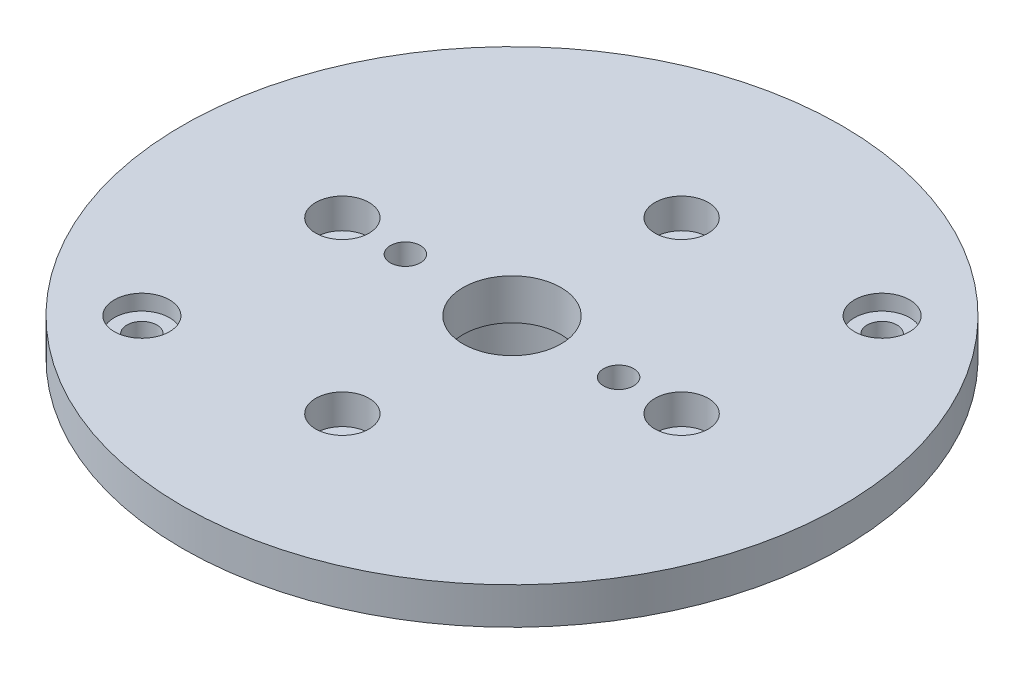
from build123d import *

# Parameters (mm, degrees)
SKETCH1_R               = 20
SKETCH1_R_2             = 7.5
BOSS_EXTRUDE1_DEPTH     = 12
SKETCH9_W               = 1.3
SKETCH9_H               = 0.7
SKETCH12_W              = 14
SKETCH12_H              = 3.8
SKETCH5_R               = 0.8
CUT_EXTRUDE2_DEPTH      = 50.558046773
SKETCH11_R              = 2.75
SKETCH11_R_2            = 1.5
CUT_EXTRUDE4_DEPTH      = 3.1
SKETCH14_W              = 4.95
SKETCH14_H              = 4.2
CUT_EXTRUDE5_DEPTH      = 50.558046773
CUT_EXTRUDE5_DEPTH_BACK = 1.6
SKETCH15_R              = 2.85
SKETCH7_R               = 1.55
CUT_EXTRUDE3_DEPTH      = 3
SKETCH16_R              = 1.55
CUT_EXTRUDE6_DEPTH      = 50.195121709
SKETCH17_R              = 1.55
CUT_EXTRUDE7_DEPTH      = 50.195121709
SKETCH18_R              = 1.5
CUT_EXTRUDE8_DEPTH      = 50.558046773


with BuildPart() as part:
    # Sketch1 → Boss-Extrude1 (new body)
    with BuildSketch(Plane(origin=(0, 0, 0), x_dir=(1, 0, 0), z_dir=(0, 1, 0))):
        with Locations(Location((0, 0, 0), (0, 0, 270))):
            Circle(SKETCH1_R)
        with Locations(Location((0, 0, 0), (0, 0, 270))):
            Circle(SKETCH1_R_2, mode=Mode.SUBTRACT)
    extrude(amount=BOSS_EXTRUDE1_DEPTH)

    # Sketch9 → Cut-Revolve3 (revolve, cut)
    with BuildSketch(Plane.XY, mode=Mode.PRIVATE) as cut_revolve3_sk:
        with Locations((14.4, 0.35)):
            Rectangle(SKETCH9_W, SKETCH9_H)
    revolve(cut_revolve3_sk.sketch.rotate(Axis((0, -3.122441051, 0), (0, 1, 0)), 90), axis=Axis((0, -3.122441051, 0), (0, 1, 0)), mode=Mode.SUBTRACT)

    # Sketch12 → Revolve1 (revolve)
    with BuildSketch(Plane.XY, mode=Mode.PRIVATE) as revolve1_sk:
        with Locations((27, 10.1)):
            Rectangle(SKETCH12_W, SKETCH12_H)
    revolve(revolve1_sk.sketch.rotate(Axis((0, 0, 0), (0, 1, 0)), 90), axis=Axis((0, 0, 0), (0, 1, 0)))

    # Sketch5 → Cut-Extrude2 (cut, through all)
    with BuildSketch(Plane(origin=(0, 12, 0), x_dir=(1, 0, 0), z_dir=(0, 1, 0))):
        with Locations(Location((11, 0, 0), (0, 0, 270))):
            Circle(SKETCH5_R)
        with Locations(Location((-11, 0, 0), (0, 0, 270))):
            Circle(SKETCH5_R)
    extrude(amount=-CUT_EXTRUDE2_DEPTH, mode=Mode.SUBTRACT)

    # Sketch11 → Cut-Extrude4 (cut)
    # profile 1 of 4: a face of its own
    with BuildSketch(Plane(origin=(0, 12, 0), x_dir=(1, 0, 0), z_dir=(0, 1, 0))):
        with Locations(Location((-17.5, 0, 0), (0, 0, 270))):
            Circle(SKETCH11_R)
        with Locations(Location((-17.5, 0, 0), (0, 0, 270))):
            Circle(SKETCH11_R_2, mode=Mode.SUBTRACT)
    # profile 2 of 4: a face of its own
    with BuildSketch(Plane(origin=(0, 12, 0), x_dir=(1, 0, 0), z_dir=(0, 1, 0))):
        with Locations(Location((0, 17.5, 0), (0, 0, 270))):
            Circle(SKETCH11_R)
        with Locations(Location((0, 17.5, 0), (0, 0, 270))):
            Circle(SKETCH11_R_2, mode=Mode.SUBTRACT)
    # profile 3 of 4: a face of its own
    with BuildSketch(Plane(origin=(0, 12, 0), x_dir=(1, 0, 0), z_dir=(0, 1, 0))):
        with Locations(Location((17.5, 0, 0), (0, 0, 270))):
            Circle(SKETCH11_R)
        with Locations(Location((17.5, 0, 0), (0, 0, 270))):
            Circle(SKETCH11_R_2, mode=Mode.SUBTRACT)
    # profile 4 of 4: a face of its own
    with BuildSketch(Plane(origin=(0, 12, 0), x_dir=(1, 0, 0), z_dir=(0, 1, 0))):
        with Locations(Location((0, -17.5, 0), (0, 0, 270))):
            Circle(SKETCH11_R)
        with Locations(Location((0, -17.5, 0), (0, 0, 270))):
            Circle(SKETCH11_R_2, mode=Mode.SUBTRACT)
    extrude(amount=-CUT_EXTRUDE4_DEPTH, mode=Mode.SUBTRACT)

    # Sketch14 → Revolve2 (revolve)
    with BuildSketch(Plane.XY, mode=Mode.PRIVATE) as revolve2_sk:
        with Locations((7.525, 9.9)):
            Rectangle(SKETCH14_W, SKETCH14_H)
    revolve(revolve2_sk.sketch.rotate(Axis((0, -21.99633859, 0), (0, 1, 0)), 90), axis=Axis((0, -21.99633859, 0), (0, 1, 0)))

    # Sketch15 → Cut-Extrude5 (cut, two sides: drawn at the far end of the back side and taken through both)
    with BuildSketch(Plane(origin=(0, 12, 0), x_dir=(1, 0, 0), z_dir=(0, 1, 0)).offset(-CUT_EXTRUDE5_DEPTH_BACK)):
        with Locations(Location((-19.091883092, -19.091883092, 0), (0, 0, 90))):
            Circle(SKETCH15_R)
        with Locations(Location((19.091883092, 19.091883092, 0), (0, 0, 90))):
            Circle(SKETCH15_R)
    extrude(amount=CUT_EXTRUDE5_DEPTH + CUT_EXTRUDE5_DEPTH_BACK, mode=Mode.SUBTRACT)

    # Sketch7 → Cut-Extrude3 (cut)
    with BuildSketch(Plane(origin=(0, 12, 0), x_dir=(1, 0, 0), z_dir=(0, 1, 0))):
        with Locations(Location((11, 0, 0), (0, 0, 270))):
            Circle(SKETCH7_R)
        with Locations(Location((-11, 0, 0), (0, 0, 270))):
            Circle(SKETCH7_R)
    extrude(amount=-CUT_EXTRUDE3_DEPTH, mode=Mode.SUBTRACT)

    # Sketch16 → Cut-Extrude6 (cut, through all)
    with BuildSketch(Plane(origin=(0, 10.4, 0), x_dir=(1, 0, 0), z_dir=(0, 1, 0))):
        with Locations(Location((-19.091883092, -19.091883092, 0), (0, 0, 270))):
            Circle(SKETCH16_R)
    extrude(amount=-CUT_EXTRUDE6_DEPTH, mode=Mode.SUBTRACT)

    # Sketch17 → Cut-Extrude7 (cut, through all)
    with BuildSketch(Plane(origin=(0, 10.4, 0), x_dir=(1, 0, 0), z_dir=(0, 1, 0))):
        with Locations(Location((19.091883092, 19.091883092, 0), (0, 0, 270))):
            Circle(SKETCH17_R)
    extrude(amount=-CUT_EXTRUDE7_DEPTH, mode=Mode.SUBTRACT)

    # Sketch18 → Cut-Extrude8 (cut, through all)
    with BuildSketch(Plane(origin=(0, 12, 0), x_dir=(1, 0, 0), z_dir=(0, 1, 0))):
        with Locations(Location((0, 17.5, 0), (0, 0, 270))):
            Circle(SKETCH18_R)
        with Locations(Location((-17.5, 0, 0), (0, 0, 270))):
            Circle(SKETCH18_R)
        with Locations(Location((0, -17.5, 0), (0, 0, 270))):
            Circle(SKETCH18_R)
        with Locations(Location((17.5, 0, 0), (0, 0, 270))):
            Circle(SKETCH18_R)
    extrude(amount=-CUT_EXTRUDE8_DEPTH, mode=Mode.SUBTRACT)


solid = part.part
